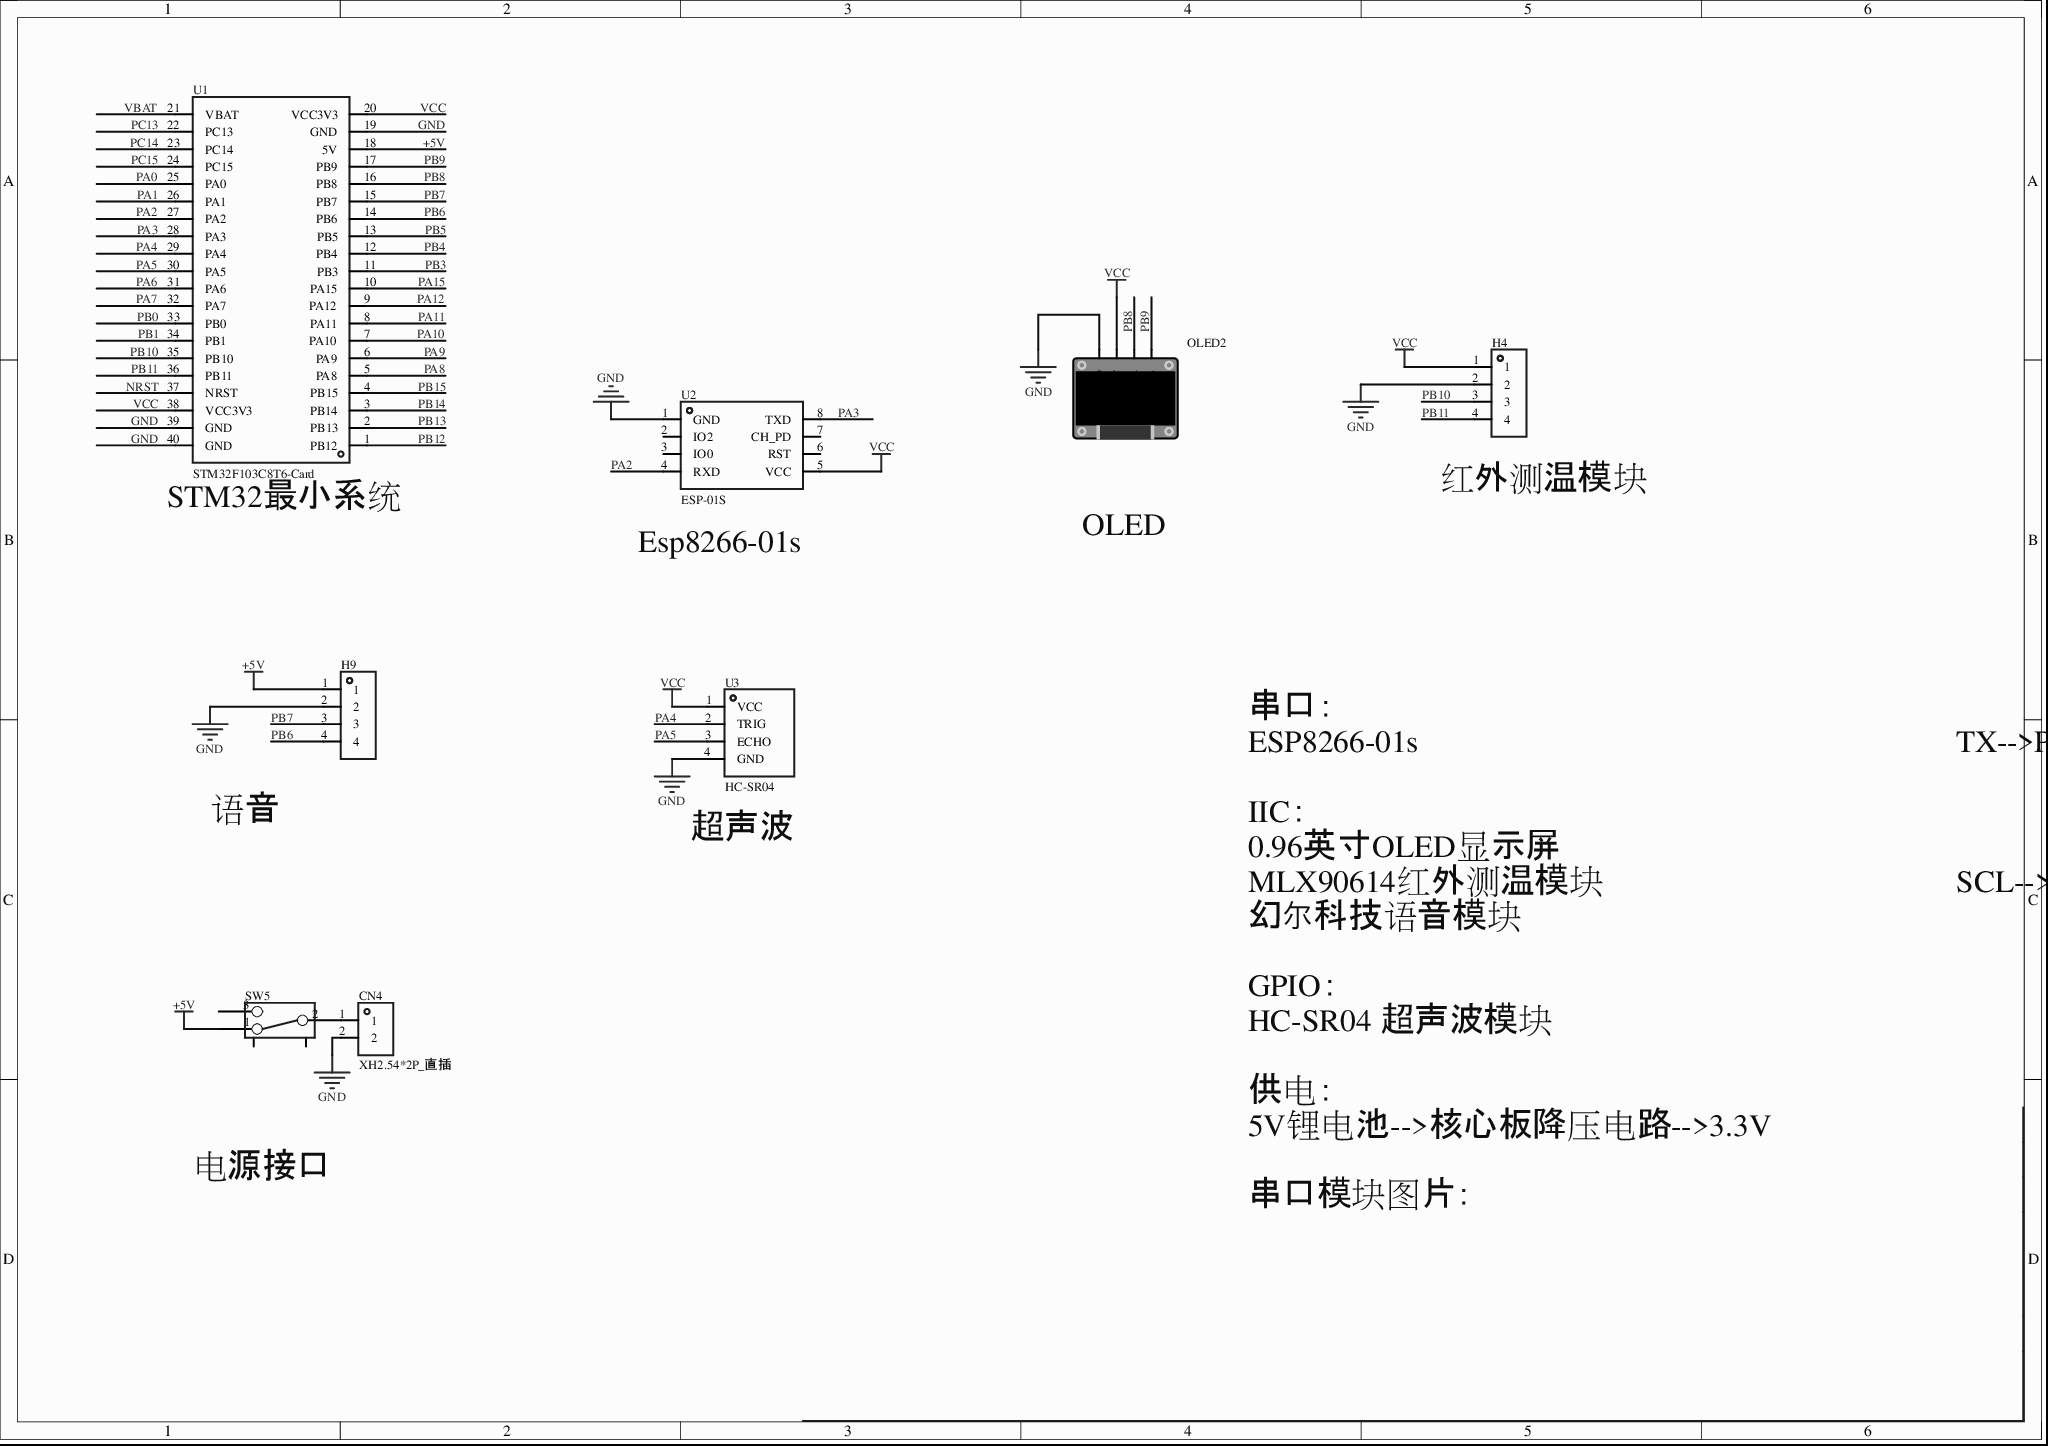
[diagram p0: MISC51851-3.schdoc]
# Altium project MISC51851-2.PrjPcb
1 sheet, 8 parts. Net scope: global (net labels, ports and power ports of the same name join across sheets).
Board file: MISC51851.pcbdoc

## Sheet MISC51851-3.schdoc
size 297 x 209 mm; Version: V1.0; @Project Name: MISC51851; @Page Count: 1; @Update Date: 2026-05-06; @Create Date: 2026-05-06; @Schematic Name: MISC51851; @Page No: 1; @Create Time: 23:22:16; @Update Time: 17:32:40; @Board Name: MISC51851

### Parts
CN4  XH2.54*2P_直插  [CONN-TH_2P-P2.50-XH2.54-2P]
H4  (no value)  [HDR-TH_4P-P2.54-V-F]
H9  (no value)  [HDR-TH_4P-P2.54-V-F]
OLED2  (no value)  [0.96OLED_4P]
SW5  (no value)  [拨动开关]
U1  STM32F103C8T6-Card  [CONN-TH_L53.3-W22.9_STM32F103C8T6-CARD]
U2  ESP-01S  [WIFIM-TH_ESP-01S]
U3  HC-SR04  [TH_HC-SR04V]

### Nets
+5V: H9.1 SW5.1 U1.18(5V)
GND: CN4.2 H4.2 H9.2 OLED2.1(GND) U1.19(GND) U1.39(GND) U1.40(GND) U2.1(GND) U3.4(GND)
VCC: H4.1 OLED2.2(VCC) U1.20(VCC3V3) U1.38(VCC3V3) U2.5(VCC) U3.1(VCC)
NRST: U1.37(NRST)
PA0: U1.25(PA0)
PA1: U1.26(PA1)
PA2: U1.27(PA2) U2.4(RXD)
PA3: U1.28(PA3) U2.8(TXD)
PA4: U1.29(PA4) U3.2(TRIG)
PA5: U1.30(PA5) U3.3(ECHO)
PA6: U1.31(PA6)
PA7: U1.32(PA7)
PA8: U1.5(PA8)
PA9: U1.6(PA9)
PA10: U1.7(PA10)
PA11: U1.8(PA11)
PA12: U1.9(PA12)
PA15: U1.10(PA15)
PB0: U1.33(PB0)
PB1: U1.34(PB1)
PB3: U1.11(PB3)
PB4: U1.12(PB4)
PB5: U1.13(PB5)
PB6: H9.4 U1.14(PB6)
PB7: H9.3 U1.15(PB7)
PB8: OLED2.3(SCL) U1.16(PB8)
PB9: OLED2.4(SDA) U1.17(PB9)
PB10: H4.3 U1.35(PB10)
PB11: H4.4 U1.36(PB11)
PB12: U1.1(PB12)
PB13: U1.2(PB13)
PB14: U1.3(PB14)
PB15: U1.4(PB15)
PC13: U1.22(PC13)
PC14: U1.23(PC14)
PC15: U1.24(PC15)
VBAT: U1.21(VBAT)
NetCN4_1: CN4.1 SW5.2

Not connected (* = marked no-connect by the designer): SW5 3 4 5; U2 2(IO2)* 3(IO0)* 6(RST)* 7(CH_PD)*

### Notes on the sheet
- (near U1) STM32最小系统
- (near H4) 红外测温模块
- (near U2) Esp8266-01s
- OLED
- 串口：
  ESP8266-01s				TX-->PA3 ;  Rx-->PA2 	(串口2）
  IIC：
  0.96英寸OLED显示屏				SCL-->PB8 ;  SDA-->PB9
  MLX90614红外测温模块			SCL-->PB10 ;  SDA-->PB11
  幻尔科技语音模块					SCL-->PB86;  SDA-->PB7
  GPIO：
  HC-SR04 超声波模块				TRIG-->PA4; ECHO-->PA5
  供电：
  5V锂电池-->核心板降压电路-->3.3V
  串口模块图片：
- 语音
- (near U3) 超声波
- 电源接口

### Library data of the parts
CN4 = XH2.54*2P_直插: 3D Model: 325c595e30db4df8abe76612dd40b0fa0819f05c4eef4c71ace90d822a990e87; 3D Model Transform: 295.275,228.346,0,180,0,0,-0.002,-20.079,-137.795; AddInBom: yes; Device: XH2.54*2P_直插; Symbol: XH2.54*2P_直插; LCSC Part Name: XH2.54*2P_直插; Supplier Part: C9900008615; Manufacturer Part: XH2.54*2P_直插; Supplier Footprint: XH2.54_2P; JLCPCB Part Class: Extended Part; Supplier: LCSC; FootprintName: CONN-TH_2P-P2.50-XH2.54-2P; ConvertToPcb: yes; ModelName: CONN-TH_2P-P2.50-XH2.54-2P
H4 = HDR-F_2.54_1x4P: Symbol: 2.54-1*4P母; ConvertToPcb: yes; ModelId: d187812051054f85879fcaa51a310d8e0819f05c4eef4c71ace90d822a990e87; ModelTransform: 419.6842,98.464,0,0,0,0,0,0,-118.11; Device: HDR-F_2.54_1x4P; FootprintName: HDR-TH_4P-P2.54-V-F; AddInBom: yes; SupplierPart: C2718488; Supplier Footprint: 插件; ModelName: HDR-TH_4P-P2.54-V-F
H9 = HDR-F_2.54_1x4P: Symbol: 2.54-1*4P母; 3D Model: d187812051054f85879fcaa51a310d8e0819f05c4eef4c71ace90d822a990e87; 3D Model Transform: 419.6842,98.464,0,0,0,0,0,0,-118.11; ConvertToPcb: yes; Device: HDR-F_2.54_1x4P; Supplier Part: C2718488; Supplier Footprint: 插件; FootprintName: HDR-TH_4P-P2.54-V-F; AddInBom: yes; ModelName: HDR-TH_4P-P2.54-V-F
OLED2 = 0.96OLED模块_4P: 3D Model: 79c000fdb68d45a296c2e9bedf4f9055; 3D Model Transform: 1393.69792,1318.895,0,0,0,0,0,-560.079,-137.795; ConvertToPcb: yes; Symbol: 0.96OLED模块_4P; Device: 0.96OLED模块_4P; Supplier Footprint: 插件; AddInBom: yes; FootprintName: 0.96OLED_4P; ModelName: 0.96OLED_4P
SW5 = 拨动开关_正: ConvertToPcb: yes; ModelId: 4321fe59a4074cbfb4989553f297c68f0819f05c4eef4c71ace90d822a990e87; ModelName: SW-TH_SS-12D02-VG4; ModelTransform: 370.09,208.7,472.35,0,0,0,0,0,-110; Device: 拨动开关_正; Symbol: 拨动开关; FootprintName: 拨动开关; AddInBom: yes; Supplier Footprint: 插件
U1 = STM32F103C8T6-Card: AddInBom: yes; Device: STM32F103C8T6-Card; Symbol: STM32F103C8T6-CARD; FootprintName: CONN-TH_L53.3-W22.9_STM32F103C8T6-CARD; LCSC Part Name: STM32F103C8T6-Card; SupplierPart: C9900077949; ManufacturerPart: STM32F103C8T6-Card; Supplier Footprint: 插件; Supplier: LCSC; ConvertToPcb: yes
U2 = ESP-01S_C111009: 3D Model: eb7175da78ae48b3b1568cfe3027405f0819f05c4eef4c71ace90d822a990e87; 3D Model Transform: 582.676,976.37608,0,0,0,0,0,388.346,-118.11; AddInBom: yes; Symbol: ESP-01S; Device: ESP-01S_C111009; LCSC Part Name: ESP-01S; Supplier Part: C111009; Manufacturer Part: ESP-01S; Supplier Footprint: -; JLCPCB Part Class: Extended Part; Supplier: LCSC; ConvertToPcb: yes; FootprintName: WIFIM-TH_ESP-01S; ModelName: WIFIM-TH_ESP-01S
U3 = HC-SR04: Manufacturer: Universal Microelectronics; AddInBom: yes; Symbol: HC-SR04; Device: HC-SR04; LCSC Part Name: HC-SR04; SupplierPart: C19857336; ManufacturerPart: HC-SR04; Supplier Footprint: -; JLCPCB Part Class: 扩展库; Datasheet: https://atta.szlcsc.com/upload/public/pdf/source/20240122/47B8E374E428935B7962A2189EF91AAC.pdf; Supplier: LCSC; ConvertToPcb: yes; FootprintName: TH_HC-SR04V